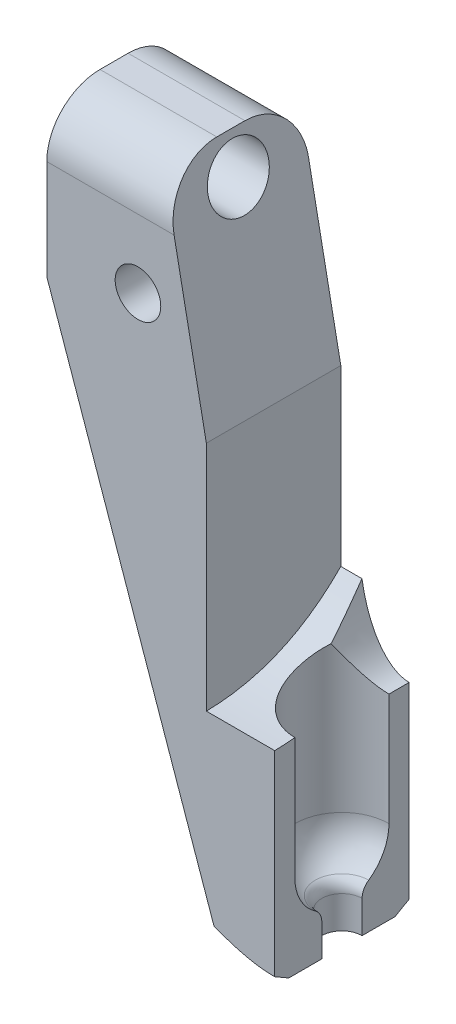
SolidWorks part; units mm, degrees
ref_plane "Front Plane" through (0, 0, 0) normal (0, 0, 1) x (1, 0, 0)
ref_plane "Top Plane" through (0, 0, 0) normal (0, 1, 0) x (1, 0, 0)
ref_plane "Right Plane" through (0, 0, 0) normal (1, 0, 0) x (0, 0, -1)
sketch "Sketch1" plane through (0, 0, 0) normal (0, 0, 1) x (1, 0, 0)
  line L22 (39, -51.5036) -> (34.8377, -51.5036)
  line L23 (39, -28) -> (39, -51.5036)
  line L24 (44.6, 0) -> (39, -28)
  line L25 (60, -20.1364) -> (60, 0)
  line L26 (60, -20.1364) -> (38.9512, -80.4124)
  line L27 (60, 0) -> (44.6, 0)
  line L28 (21.0488, -80.4124) -> (0, -20.1364)
  line L29 (0, -20.1364) -> (0, 0)
  line L30 (21, -51.5036) -> (21, -28.6)
  line L31 (25.1623, -51.5036) -> (21, -51.5036)
  line L32 (21, -28.6) -> (15.3764, 0)
  line L33 (0, 0) -> (15.3764, 0)
  line L34 (37, -86) -> (23, -86)
  line L35 (25.1623, -51.5036) -> (34.8377, -51.5036)
  circle A0 centre (48, -16) radius 3
  circle A1 centre (12, -16) radius 3
  spline S0 degree 3 poles (38.9512, -80.4124) (38.741, -81.0144) (38.5334, -81.6089) (38.3309, -82.1888) knots 0 0 0 0 0.25 0.25 0.25 0.25
  spline S1 degree 3 poles (38.3309, -82.1888) (38.1284, -82.7688) (37.9302, -83.3362) (37.7441, -83.869) knots 0.25 0.25 0.25 0.25 0.5 0.5 0.5 0.5
  spline S2 degree 3 poles (37.7441, -83.869) (37.6511, -84.1355) (37.5613, -84.3926) (37.4767, -84.6348) knots 0.5 0.5 0.5 0.5 0.625 0.625 0.625 0.625
  spline S3 degree 3 poles (37.4767, -84.6348) (37.3922, -84.877) (37.3127, -85.1045) (37.2423, -85.3061) knots 0.625 0.625 0.625 0.625 0.75 0.75 0.75 0.75
  spline S4 degree 3 poles (37.2423, -85.3061) (37.1719, -85.5076) (37.1112, -85.6816) (37.0682, -85.8048) knots 0.75 0.75 0.75 0.75 0.875 0.875 0.875 0.875
  spline S5 degree 2 poles (37.0682, -85.8048) (37.0252, -85.9279) (37, -86) knots 0.875 0.875 0.875 1 1 1
  spline S6 degree 2 poles (23, -86) (22.9755, -85.9299) (22.9325, -85.8066) knots 0 0 0 0.125 0.125 0.125
  spline S7 degree 3 poles (22.9325, -85.8066) (22.911, -85.745) (22.8847, -85.6697) (22.8553, -85.5855) knots 0.125 0.125 0.125 0.125 0.1875 0.1875 0.1875 0.1875
  spline S8 degree 3 poles (22.8553, -85.5855) (22.8258, -85.5013) (22.7932, -85.4079) (22.7583, -85.3078) knots 0.1875 0.1875 0.1875 0.1875 0.25 0.25 0.25 0.25
  spline S9 degree 3 poles (22.7583, -85.3078) (22.6883, -85.1074) (22.6089, -84.8801) (22.524, -84.637) knots 0.25 0.25 0.25 0.25 0.375 0.375 0.375 0.375
  spline S10 degree 3 poles (22.524, -84.637) (22.4392, -84.3939) (22.3487, -84.1348) (22.2555, -83.8681) knots 0.375 0.375 0.375 0.375 0.5 0.5 0.5 0.5
  spline S11 degree 3 poles (22.2555, -83.8681) (22.0692, -83.3346) (21.8716, -82.7687) (21.6691, -82.1889) knots 0.5 0.5 0.5 0.5 0.75 0.75 0.75 0.75
  spline S12 degree 3 poles (21.6691, -82.1889) (21.4667, -81.6091) (21.2591, -81.0146) (21.0488, -80.4124) knots 0.75 0.75 0.75 0.75 1 1 1 1
  dimension "D1" = 36
  dimension "D2" = 16
  dimension "D3" = 12
  dimension "D4" = 12
extrude "Boss-Extrude2" add sketch "Sketch1" along normal blind 17.7
ref_plane "Plane2" through (30, 0, 0) normal (-1, 0, 0) x (0, 0, 1)
sketch "Sketch2" plane through (30, 0, 0) normal (-1, 0, 0) x (0, 0, 1)
  line L0 (11.5, -86) -> (11.5, -81.75)
  line L1 (17.7, -86) -> (0, -86) construction
  line L2 (15.0441, -75) -> (15.0441, -57.48)
  line L3 (102, 6.2) -> (84.4804, 6.2)
  line L4 (113, 2.65) -> (108.7541, 2.65)
  line L5 (11.5, -86) -> (8.85, -86)
  line L6 (8.85, -86) -> (8.85, -57.48)
  line L7 (8.85, -57.48) -> (15.0441, -57.48)
  arc A0 (107.1067, 3.5159) -> (108.7541, 2.65) centre (108.7541, 4.65) ccw
  arc A1 (107.1067, 3.5159) -> (102, 6.2) centre (102, 0) ccw
  arc A2 (11.5, -81.75) -> (12.3644, -80.1037) centre (13.5, -81.75) cw
  arc A3 (12.3644, -80.1037) -> (15.0441, -75) centre (8.8441, -75) ccw
  point P8 (8.85, -86)
  dimension "D1" = 4.25
  dimension "D2" = 2
  dimension "D3" = 6.2
  dimension "D4" = 28.52
  dimension "D5" = 17.52
  dimension "D6" = 2.65
revolve "Cut-Revolve2" cut sketch "Sketch2" angle 360 about L6
sketch "Sketch3" plane through (30, 0, 0) normal (-1, 0, 0) x (0, 0, 1)
  line L0 (17.7, -20.1364) -> (17.7, -80.4124) construction
  line L2 (0, -51.5036) -> (17.7, -51.5036)
  line L3 (17.7, -51.5036) -> (17.7, -59.1523)
  line L4 (2.6559, -57.48) -> (15.0441, -57.48) construction
  spline S0 degree 2 poles (17.7, -59.1523) (7.3354, -59.0089) (0, -51.5036) knots 0 0 0 1 1 1
extrude "Cut-Extrude1" cut sketch "Sketch3" against normal up to surface and the other way up to surface up to face at (39, -39.7518, 8.85) other way up to face at (21, -40.0518, 8.85)
sketch "Sketch4" plane through (30, 0, 0) normal (-1, 0, 0) x (0, 0, 1)
  line L0 (4.1824, -56.4823) -> (-7.4784, -54.9866)
ref_plane "Plane4" through (0, 0, 8.85) normal (0, 0, -1) x (-1, 0, 0)
sketch "Sketch6" plane through (0, 0, 8.85) normal (0, 0, -1) x (-1, 0, 0)
  line L1 (-30, -56.4823) -> (-30, -54.9866) construction
  ellipse E0 centre (-30, -47.9683) end of major axis (-30, -35.7103) minor radius 6.4919
extrude "Cut-Extrude2" cut sketch "Sketch6" along normal blind 48.7
sketch "Sketch7" plane through (0, 0, 0) normal (0, 1, 0) x (1, 0, 0)
  circle A0 centre (30, -8.85) radius 6.1941
extrude "Cut-Extrude3" cut sketch "Sketch7" against normal blind 60.7
ref_plane "Plane5" through (6, 0, 0) normal (-1, 0, 0) x (0, 0, 1)
sketch "Sketch8" plane through (6, 0, 0) normal (-1, 0, 0) x (0, 0, 1)
  line L0 (17.7, 0) -> (0, 0) construction
  line L1 (17.7, -86) -> (0, -86) construction
  circle A0 centre (8.85, -5) radius 4
  point P7 (8.85, -86)
  dimension "D1" = 8
  dimension "D2" = 5
extrude "Cut-Extrude4" cut sketch "Sketch8" against normal blind 48
fillet "Fillet1" radius 7 4 edges at (52.3, 0, 17.7) (52.3, 0, 0) (7.6882, 0, 0) (7.6882, 0, 17.7)
sketch "Sketch10" plane through (0, -86, 0) normal (0, -1, 0) x (1, 0, 0)
  circle A0 centre (30, 8.85) radius 7
  dimension "D1" = 14
extrude "Cut-Extrude5" cut sketch "Sketch10" against normal blind 48 draft 60 flip side to cut
ref_plane "Plane6" through (0, -5, 0) normal (0, 1, 0) x (1, 0, 0)
sketch "Sketch12" plane through (0, 0, 17.7) normal (0, 0, 1) x (1, 0, 0)
  line L0 (30, -86) -> (30, 13.7307)
  line L1 (23, -86) -> (37, -86) construction
  line L2 (30, 13.7307) -> (80.8166, 10.061)
  line L3 (80.8166, 10.061) -> (70.6813, -110.3401)
  line L4 (70.6813, -110.3401) -> (30, -86)
extrude "Cut-Extrude7" cut sketch "Sketch12" against normal blind 44
